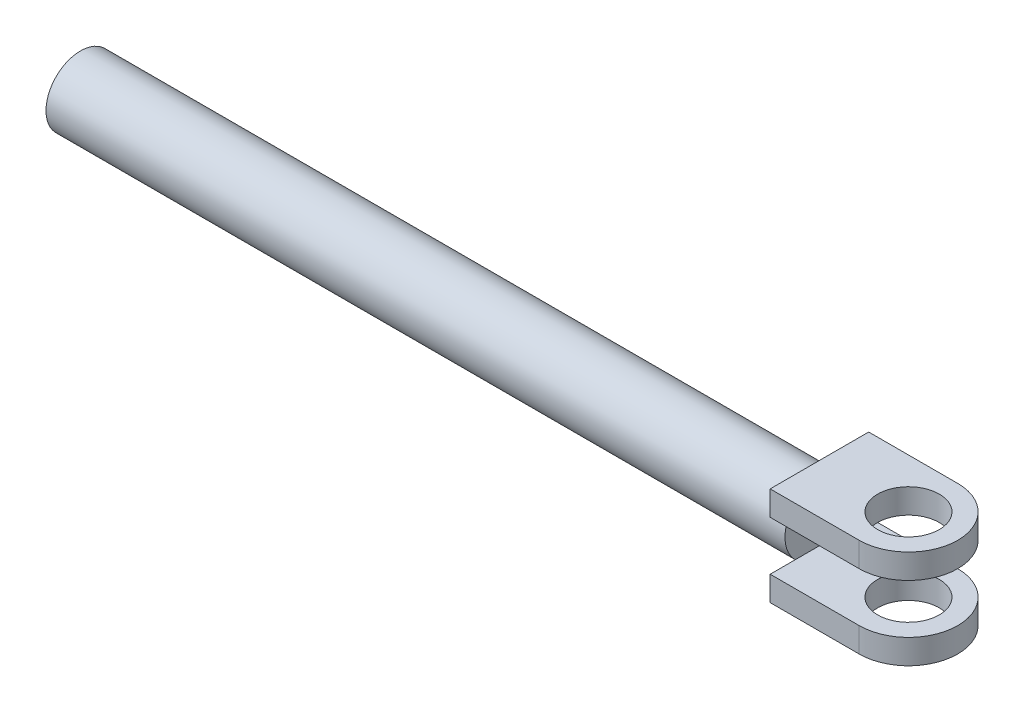
from build123d import *

# Parameters (mm, degrees)
SKETCH1_R           = 12.5
BOSS_EXTRUDE1_DEPTH = 10
SKETCH2_R           = 14
BOSS_EXTRUDE2_DEPTH = 300


with BuildPart() as part:
    # Sketch1 → Boss-Extrude1 (new body)
    with BuildSketch(Plane(origin=(0, 0, 0), x_dir=(1, 0, 0), z_dir=(0, 1, 0))):
        with BuildLine():
            Line((36.142857143, 20), (72.285714286, 20))
            ThreePointArc((72.285714286, 20), (92.285714286, 0), (72.285714286, -20))
            Line((72.285714286, -20), (36.142857143, -20))
            Line((36.142857143, -20), (36.142857143, 20))
        make_face()
        with Locations(Location((72.285714286, 0, 0), (0, 0, 270))):
            Circle(SKETCH1_R, mode=Mode.SUBTRACT)
    boss_extrude1 = extrude(amount=BOSS_EXTRUDE1_DEPTH)

    # Sketch2 → Boss-Extrude2 (add)
    with BuildSketch(Plane.ZY.offset(-36.142857143)):
        with Locations(Location((0, -10, 0), (0, 0, 134.415308597))):
            Circle(SKETCH2_R)
    extrude(amount=BOSS_EXTRUDE2_DEPTH)

    # Mirror1: Boss-Extrude1 across plane
    add(boss_extrude1.mirror(Plane(origin=(0, -10, 0), x_dir=(0, 0, 1), z_dir=(0, -1, 0))))


solid = part.part
